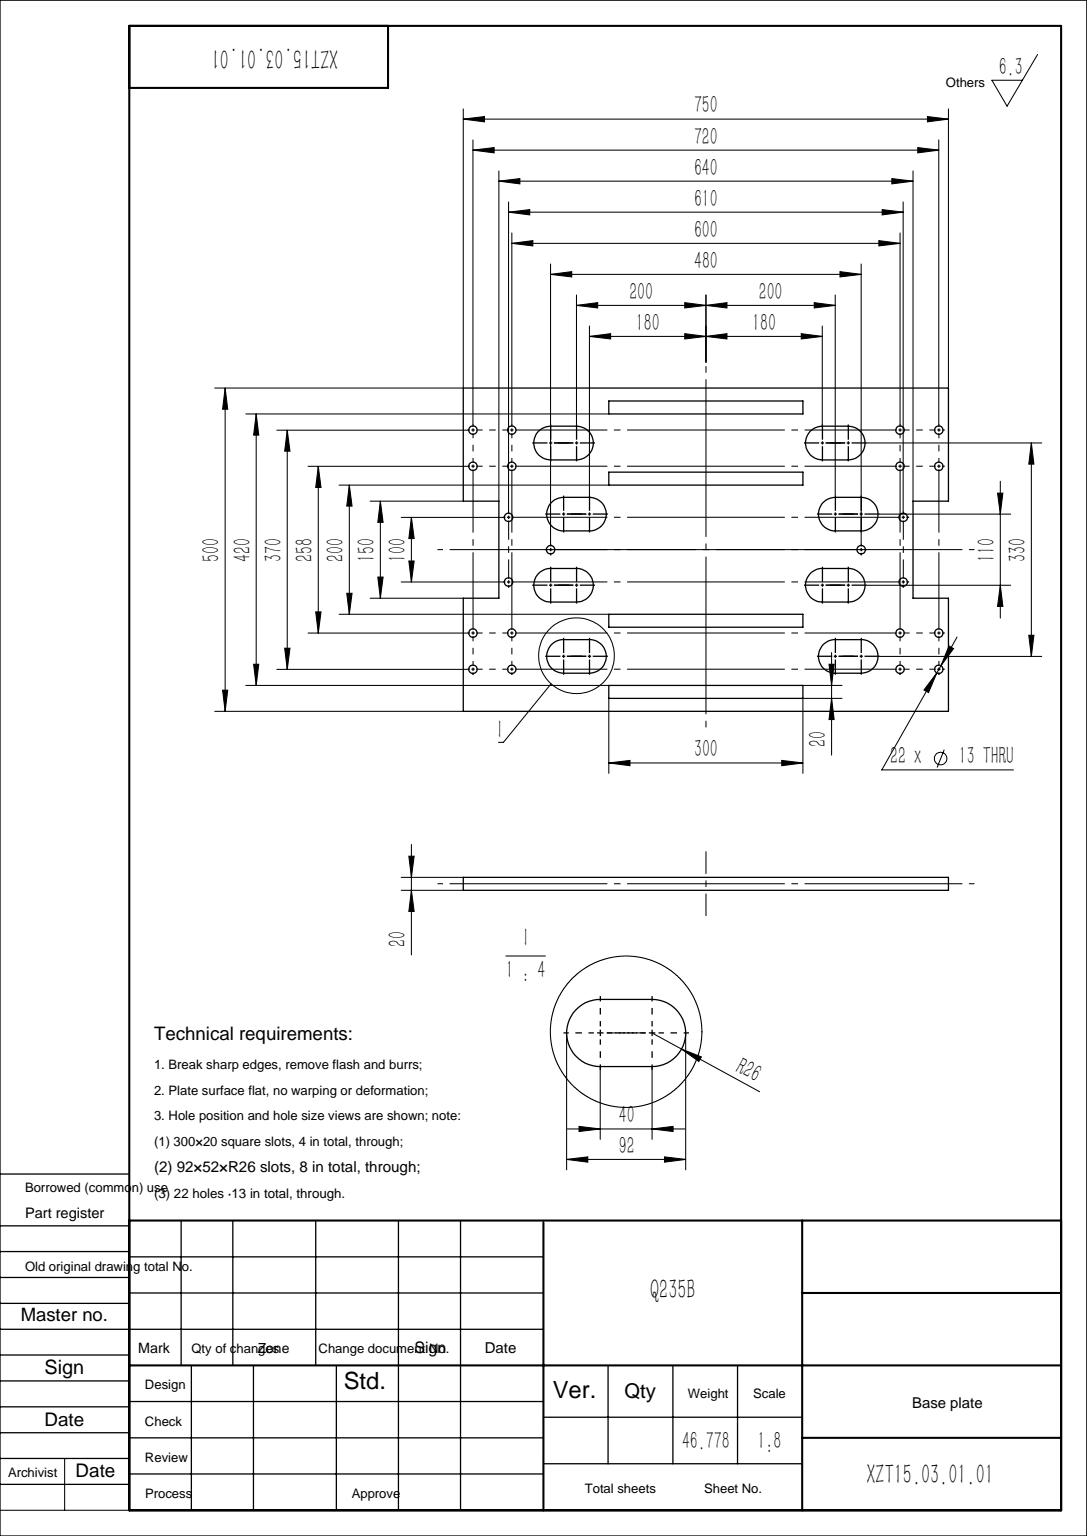
SolidWorks part; units mm, degrees
material "Q235B"
ref_plane "Front Plane" through (0, 0, 0) normal (0, 0, 1) x (1, 0, 0)
ref_plane "Top Plane" through (0, 0, 0) normal (0, 1, 0) x (1, 0, 0)
ref_plane "Right Plane" through (0, 0, 0) normal (1, 0, 0) x (0, 0, -1)
sketch "Sketch1" plane through (0, 0, 0) normal (0, 1, 0) x (1, 0, 0)
  line L0 (0, 0) -> (0, 250) construction
  line L1 (375, -250) -> (-375, -250)
  line L2 (375, -250) -> (375, 250)
  line L3 (375, 250) -> (-375, 250)
  line L4 (-375, -250) -> (-375, 250)
  line L5 (375, -250) -> (-375, 250) construction
  line L6 (375, 250) -> (-375, -250) construction
  line L7 (-320, -75) -> (-430, -75)
  line L8 (-320, -75) -> (-320, 75)
  line L9 (-320, 75) -> (-430, 75)
  line L10 (-430, -75) -> (-430, 75)
  line L11 (-320, -75) -> (-430, 75) construction
  line L12 (-320, 75) -> (-430, -75) construction
  line L13 (0, 0) -> (375, 0) construction
  line L14 (150, -120) -> (-150, -100) construction
  line L15 (150, 210) -> (-150, 210)
  line L16 (150, 210) -> (150, 230)
  line L17 (150, 230) -> (-150, 230)
  line L18 (-150, 210) -> (-150, 230)
  line L19 (150, 210) -> (-150, 230) construction
  line L20 (150, 230) -> (-150, 210) construction
  line L21 (150, 100) -> (-150, 100)
  line L22 (150, 100) -> (150, 120)
  line L23 (150, 120) -> (-150, 120)
  line L24 (-150, 100) -> (-150, 120)
  line L25 (150, 100) -> (-150, 120) construction
  line L26 (150, 120) -> (-150, 100) construction
  line L27 (150, -100) -> (-150, -120) construction
  line L28 (150, -230) -> (-150, -210) construction
  line L29 (150, -210) -> (-150, -230) construction
  line L30 (-150, -100) -> (-150, -120)
  line L31 (150, -120) -> (-150, -120)
  line L32 (150, -100) -> (150, -120)
  line L33 (150, -100) -> (-150, -100)
  line L34 (-150, -210) -> (-150, -230)
  line L35 (150, -230) -> (-150, -230)
  line L36 (150, -210) -> (150, -230)
  line L37 (150, -210) -> (-150, -210)
  line L38 (320, 75) -> (430, -75) construction
  line L39 (320, -75) -> (430, 75) construction
  line L40 (430, -75) -> (430, 75)
  line L41 (320, 75) -> (430, 75)
  line L42 (320, -75) -> (320, 75)
  line L43 (320, -75) -> (430, -75)
  point P0 (0, 0)
  point P5 (-375, 0)
  point P14 (0, 220)
  point P19 (0, 110)
  point P32 (0, -110)
  point P33 (0, -220)
  dimension "D1" = 500
  dimension "D2" = 750
  dimension "D3" = 150
  dimension "D4" = 110
  dimension "D5" = 20
  dimension "D6" = 300
  dimension "D7" = 200
  dimension "D8" = 420
extrude "Boss-Extrude1" add sketch "Sketch1" along normal blind 20 contours L43 L42 L41 L2 L3 L4 L9 L8 L7 L1 L37 L36 L35 L34 L33 L32 L31 L30 L15 L18 L17 L16 L21 L24 L23 L22
hole_wizard "Ø13.0 (13) Diameter Hole1" positions "Sketch2" profile "Sketch3" hole size "Ø13.0" standard "GB" end condition up to next
sketch "Sketch2" plane through (0, 20, 0) normal (0, 1, 0) x (1, 0, 0)
  line L0 (-240, 0) -> (0, 0) construction
  line L1 (0, 0) -> (0, 250) construction
  line L2 (375, 250) -> (-375, 250) construction
  line L4 (-360, 129) -> (-300, 129) construction
  line L5 (-360, 129) -> (-360, 185) construction
  line L6 (-360, -129) -> (-360, -185) construction
  line L7 (-360, -129) -> (-300, -129) construction
  line L8 (360, -129) -> (300, -129) construction
  line L9 (360, -129) -> (360, -185) construction
  line L10 (360, 129) -> (360, 185) construction
  line L11 (360, 129) -> (300, 129) construction
  point P0 (-360, 129)
  point P2 (-305, 50)
  point P4 (-240, 0)
  point P19 (-300, 129)
  point P20 (-300, 185)
  point P21 (-360, 185)
  point P26 (-360, -129)
  point P27 (-360, -185)
  point P28 (-300, -129)
  point P29 (-300, -185)
  point P30 (-305, -50)
  point P38 (360, -129)
  point P39 (300, -129)
  point P40 (360, -185)
  point P41 (360, 129)
  point P42 (360, 185)
  point P43 (300, 129)
  point P44 (305, -50)
  point P45 (300, -185)
  point P46 (300, 185)
  point P47 (240, 0)
  point P48 (305, 50)
  dimension "D1" = 480
  dimension "D2" = 610
  dimension "D5" = 90
  dimension "D6" = 60
  dimension "D7" = 56
  dimension "D8" = 600
  dimension "D9" = 258
  dimension "D10" = 100
  dimension "D3" = 2
  dimension "D4" = 2
sketch "Sketch3" plane through (-360, 20, -129) normal (1, 0, 0) x (0, 0, 1)
  line L0 (0, 0) -> (0, 20)
  line L1 (0, 20) -> (6.5, 20)
  line L2 (6.5, 20) -> (6.5, 0)
  line L5 (6.5, 0) -> (0, 0)
  line L11 (0, -6.35) -> (0, 107.95) construction
  dimension "通孔孔直径" = 13
  dimension "通孔孔深度" = 20
sketch "Sketch4" plane through (0, 20, 0) normal (0, 1, 0) x (1, 0, 0)
  line L0 (-240, 165) -> (-200, 165) construction
  line L1 (-240, 191) -> (-200, 191)
  line L2 (-240, 139) -> (-200, 139)
  line L3 (-220, 55) -> (-180, 55) construction
  line L4 (-220, 81) -> (-180, 81)
  line L5 (-220, 29) -> (-180, 29)
  line L6 (0, 250) -> (0, 0) construction
  line L7 (375, 250) -> (-375, 250) construction
  line L9 (180, 165) -> (220, 165) construction
  line L10 (180, 191) -> (220, 191)
  line L11 (180, 139) -> (220, 139)
  line L12 (200, 55) -> (240, 55) construction
  line L13 (200, 81) -> (240, 81)
  line L14 (200, 29) -> (240, 29)
  line L15 (180, -55) -> (220, -55) construction
  line L16 (180, -29) -> (220, -29)
  line L17 (180, -81) -> (220, -81)
  line L18 (200, -165) -> (240, -165) construction
  line L19 (200, -139) -> (240, -139)
  line L20 (200, -191) -> (240, -191)
  line L21 (-240, -55) -> (-200, -55) construction
  line L22 (-240, -29) -> (-200, -29)
  line L23 (-240, -81) -> (-200, -81)
  line L24 (-220, -165) -> (-180, -165) construction
  line L25 (-220, -139) -> (-180, -139)
  line L26 (-220, -191) -> (-180, -191)
  line L27 (-220, 55) -> (200, 55) construction
  line L28 (-220, 55) -> (-220, -165) construction
  arc A0 (-240, 191) -> (-240, 139) centre (-240, 165) ccw
  arc A1 (-200, 139) -> (-200, 191) centre (-200, 165) ccw
  arc A2 (-220, 81) -> (-220, 29) centre (-220, 55) ccw
  arc A3 (-180, 29) -> (-180, 81) centre (-180, 55) ccw
  arc A4 (180, 191) -> (180, 139) centre (180, 165) ccw
  arc A5 (220, 139) -> (220, 191) centre (220, 165) ccw
  arc A6 (200, 81) -> (200, 29) centre (200, 55) ccw
  arc A7 (240, 29) -> (240, 81) centre (240, 55) ccw
  arc A8 (180, -29) -> (180, -81) centre (180, -55) ccw
  arc A9 (220, -81) -> (220, -29) centre (220, -55) ccw
  arc A10 (200, -139) -> (200, -191) centre (200, -165) ccw
  arc A11 (240, -191) -> (240, -139) centre (240, -165) ccw
  arc A12 (-240, -29) -> (-240, -81) centre (-240, -55) ccw
  arc A13 (-200, -81) -> (-200, -29) centre (-200, -55) ccw
  arc A14 (-220, -139) -> (-220, -191) centre (-220, -165) ccw
  arc A15 (-180, -191) -> (-180, -139) centre (-180, -165) ccw
  point P2 (-220, 165)
  point P7 (-200, 55)
  point P24 (200, 165)
  point P29 (220, 55)
  point P38 (200, -55)
  point P43 (220, -165)
  point P52 (-220, -55)
  point P57 (-200, -165)
  dimension "D1" = 92
  dimension "D2" = 26
  dimension "D3" = 200
  dimension "D4" = 20
  dimension "D5" = 55
  dimension "D6" = 110
  dimension "D9" = 90
  dimension "D10" = 420
  dimension "D11" = 220
  dimension "D7" = 2
  dimension "D8" = 2
extrude "Cut-Extrude1" cut sketch "Sketch4" against normal up to next
